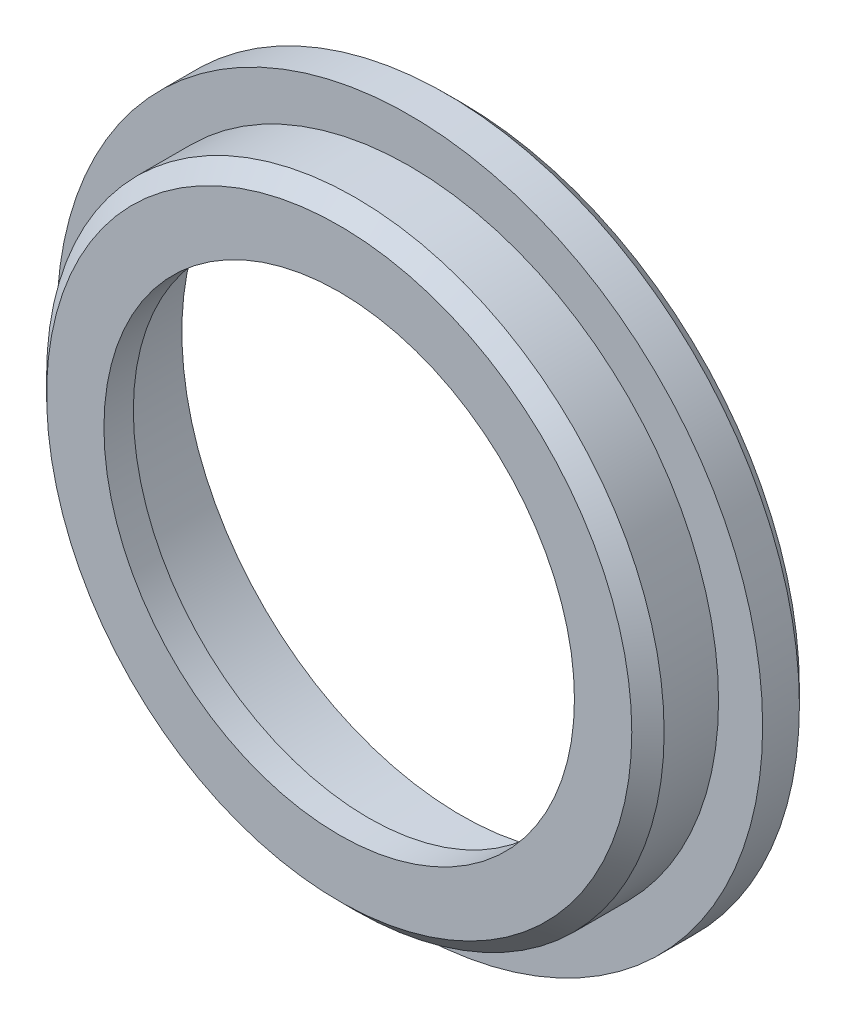
SolidWorks part; units mm, degrees
material "6061 合金"
ref_plane "前视基准面" through (0, 0, 0) normal (0, 0, 1) x (1, 0, 0)
ref_plane "上视基准面" through (0, 0, 0) normal (0, 1, 0) x (1, 0, 0)
ref_plane "右视基准面" through (0, 0, 0) normal (1, 0, 0) x (0, 0, -1)
other "Configuration Table"
sketch "草图1" plane through (0, 0, 0) normal (0, 0, 1) x (1, 0, 0)
  circle A0 centre (0, 0) radius 19
  circle A1 centre (0, 0) radius 24
  dimension "D1" = 38
  dimension "D2" = 5
extrude "凸台-拉伸1" add sketch "草图1" along normal blind 3.5
sketch "草图2" plane through (0, 0, 3.5) normal (0, 0, 1) x (1, 0, 0)
  circle A0 centre (0, 0) radius 21
  circle A1 centre (0, 0) radius 19 construction
  circle A2 centre (0, 0) radius 19
  dimension "D1" = 2
extrude "凸台-拉伸2" add sketch "草图2" along normal blind 2.8
sketch "草图3" plane through (0, 0, 6.3) normal (0, 0, 1) x (1, 0, 0)
  circle A0 centre (0, 0) radius 16
  circle A1 centre (0, 0) radius 21
  circle A2 centre (0, 0) radius 21
  dimension "D2" = 5
  dimension "D1" = 0
extrude "凸台-拉伸3" add sketch "草图3" along normal blind 2
chamfer "倒角1" distance 1.1 angle 45 2 edges at (19, 0, 6.3) (21, 0, 8.3)
chamfer "倒角2" distance 1 angle 45 1 edges at (24, 0, 0)
